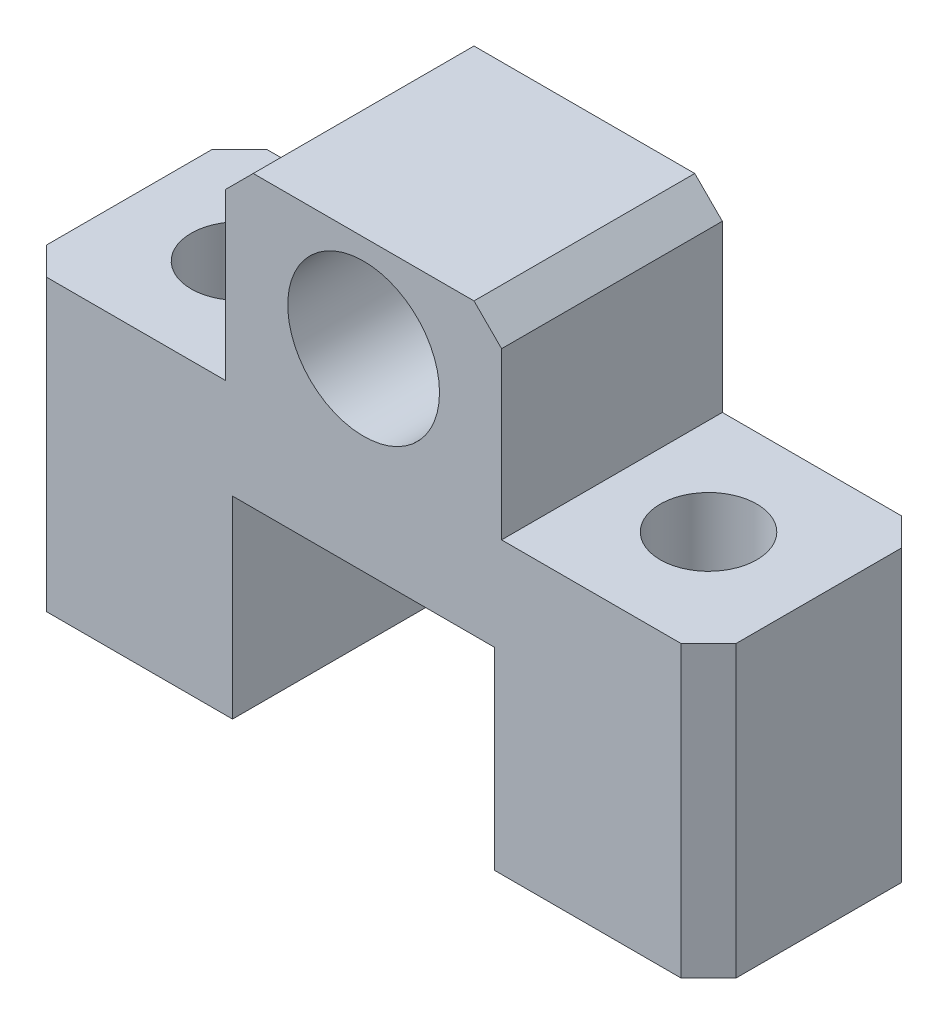
from build123d import *

# Parameters (mm, degrees)
SKETCH1_W                  = 25
SKETCH1_H                  = 17.5
BOSS_EXTRUDE1_DEPTH        = 8
SKETCH2_W                  = 7.5
SKETCH2_H                  = 7
CUT_EXTRUDE1_DEPTH         = 8
SKETCH3_W                  = 9.5
SKETCH3_H                  = 7
CUT_EXTRUDE2_DEPTH         = 18.228247154
SKETCH4_R                  = 2.75
CUT_EXTRUDE3_DEPTH         = 5
F_3_5_3_5_DIAMETER_HOLE1_D = 3.5
CHAMFER1_SIZE              = 1


with BuildPart() as part:
    # Sketch1 → Boss-Extrude1 (new body)
    with BuildSketch(Plane.XY):
        Rectangle(SKETCH1_W, SKETCH1_H)
    extrude(amount=BOSS_EXTRUDE1_DEPTH)

    # Sketch2 → Cut-Extrude1 (cut)
    with BuildSketch(Plane.XY.offset(8)):
        with Locations((8.75, 5.25)):
            Rectangle(SKETCH2_W, SKETCH2_H)
        with Locations((-8.75, 5.25)):
            Rectangle(SKETCH2_W, SKETCH2_H)
    extrude(amount=-CUT_EXTRUDE1_DEPTH, mode=Mode.SUBTRACT)

    # Sketch3 → Cut-Extrude2 (cut, through all)
    with BuildSketch(Plane.XY.offset(8)):
        with Locations((0, -5.25)):
            Rectangle(SKETCH3_W, SKETCH3_H)
    extrude(amount=-CUT_EXTRUDE2_DEPTH, mode=Mode.SUBTRACT)

    # Sketch4 → Cut-Extrude3 (cut)
    with BuildSketch(Plane.XY.offset(8)):
        with Locations((0, 5.25)):
            Circle(SKETCH4_R)
    extrude(amount=-CUT_EXTRUDE3_DEPTH, mode=Mode.SUBTRACT)

    # Ø3.5 (3.5) Diameter Hole1 (through all)
    with Locations(Plane(origin=(0, 1.75, 0), x_dir=(1, 0, 0), z_dir=(0, 1, 0))):
        with Locations((-8.5, -4), (8.5, -4)):
            Hole(F_3_5_3_5_DIAMETER_HOLE1_D / 2)

    # Chamfer1
    chamfer1_edges = [part.edges().sort_by_distance(p)[0] for p in [
        (-12.5, -3.5, 0),
        (-12.5, -3.5, 8),
        (-5, 8.75, 4),
        (5, 8.75, 4),
        (12.5, -3.5, 8),
        (12.5, -3.5, 0),
    ]]
    chamfer(chamfer1_edges, length=CHAMFER1_SIZE)


solid = part.part
